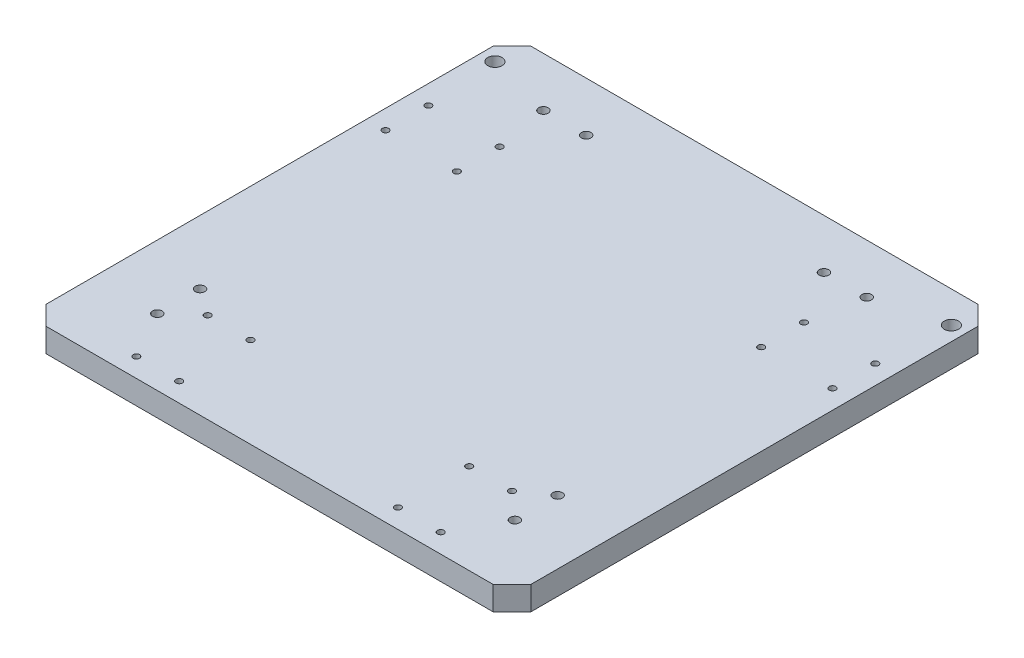
from build123d import *

# Parameters (mm, degrees)
SKETCH_1_W              = 510
SKETCH_1_H              = 510
EXTRUDE_1_DEPTH         = 12.5
HOLE_WIZARD_10_0_10_2_D = 10
HOLE_WIZARD_15_0_15_1_D = 15
HOLE_WIZARD_M8_1_D      = 6.8
CHAMFER_1_SIZE          = 20


with BuildPart() as part:
    # 草图1 → 凸台-拉伸1 (new, symmetric)
    with BuildSketch(Plane(origin=(0, 0, 0), x_dir=(1, 0, 0), z_dir=(0, 1, 0))):
        Rectangle(SKETCH_1_W, SKETCH_1_H)
    extrude(amount=EXTRUDE_1_DEPTH, both=True)

    # Ø10.0 (10) 直径孔2 (through all)
    with Locations(Plane(origin=(0, -12.5, 0), x_dir=(-1, 0, 0), z_dir=(0, -1, 0))):
        with Locations((188, -185), (188, -140), (-188, -185), (-188, -140), (170, 203), (125, 203), (-125, 203), (-170, 203)):
            Hole(HOLE_WIZARD_10_0_10_2_D / 2)

    # Ø15.0 (15) 直径孔1 (through all)
    with Locations(Plane(origin=(0, 12.5, 0), x_dir=(1, 0, 0), z_dir=(0, 1, 0))):
        with Locations((-240, -334.568738181), (-240, 222), (240, 222), (240, -307.647208852)):
            Hole(HOLE_WIZARD_15_0_15_1_D / 2)

    # M8 螺纹孔1 (through all)
    with Locations(Plane(origin=(0, -12.5, 0), x_dir=(-1, 0, 0), z_dir=(0, -1, 0))):
        with Locations((115, -160), (160, -160), (115, -235), (160, -235), (-160, -160), (-115, -160), (-115, -235), (-160, -235), (-235, 147), (-160, 147), (-160, 102), (-235, 102), (160, 147), (235, 147), (235, 102), (160, 102)):
            Hole(HOLE_WIZARD_M8_1_D / 2)

    # 倒角1
    chamfer_1_edges = [part.edges().sort_by_distance(p)[0] for p in [
        (-255, 0, -255),
        (255, 0, -255),
        (255, 0, 255),
        (-255, 0, 255),
    ]]
    chamfer(chamfer_1_edges, length=CHAMFER_1_SIZE)


solid = part.part
